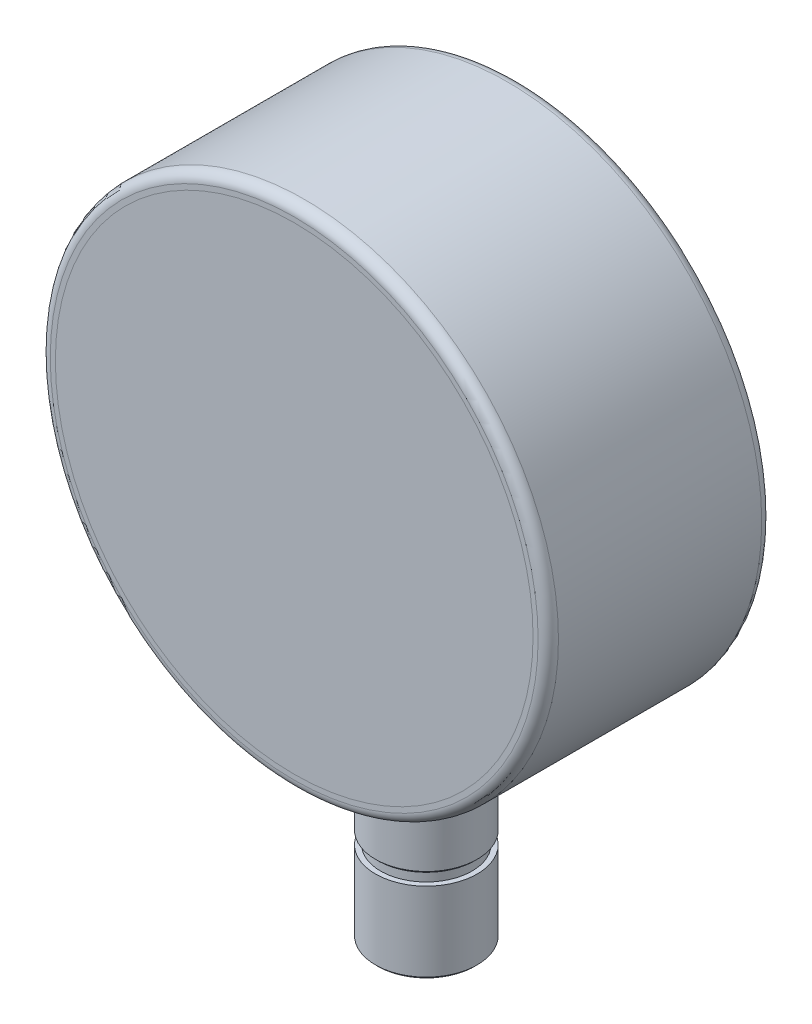
SolidWorks part; units mm, degrees
material "黄铜"
ref_plane "前视基准面" through (0, 0, 0) normal (0, 0, 1) x (1, 0, 0)
ref_plane "上视基准面" through (0, 0, 0) normal (0, 1, 0) x (1, 0, 0)
ref_plane "右视基准面" through (0, 0, 0) normal (1, 0, 0) x (0, 0, -1)
sketch "草图1" plane through (0, 0, 0) normal (0, 0, 1) x (1, 0, 0)
  circle A0 centre (0, 0) radius 50
  dimension "D" = 100
extrude "凸台-拉伸1" add sketch "草图1" along normal blind 44
fillet "圆角1" radius 2 2 edges at (50, 0, 44) (50, 0, 0)
ref_plane "基准面1" through (0, 0, 18) normal (0, 0, -1) x (-1, 0, 0)
sketch "草图2" plane through (0, 0, 18) normal (0, 0, -1) x (-1, 0, 0)
  line L0 (0, 0) -> (0, -90) construction
  line L1 (0, 0) -> (10, 0)
  line L2 (10, 0) -> (10, -70)
  line L3 (10, -70) -> (9, -70)
  line L4 (9, -70) -> (9, -72)
  line L5 (9, -72) -> (10, -72)
  line L6 (10, -72) -> (10, -88)
  line L7 (10, -88) -> (3, -88)
  line L8 (3, -88) -> (3, -90)
  line L9 (3, -90) -> (0, -90)
  line L10 (0, 0) -> (0, -90)
  dimension "B" = 90
  dimension "L" = 20
  dimension "L1" = 2
  dimension "d1" = 6
  dimension "D2" = 1
  dimension "(d)" = 20
  dimension "D3" = 2
revolve "旋转1" add sketch "草图2" angle 360 about L0
cosmetic thread "装饰螺纹线1" parameters "D2"=1
chamfer "倒角1" distance 0.5 angle 45 2 edges at (-10, -88, 18) (-10, -70, 18)
sketch "草图3" plane through (0, 0, 44) normal (0, 0, 1) x (1, 0, 0)
  circle A0 centre (0, 0) radius 47
  dimension "D1" = 94
extrude "切除-拉伸1" cut sketch "草图3" against normal blind 41
sketch "草图4" plane through (0, 0, 3) normal (0, 0, 1) x (1, 0, 0)
  line L0 (0, 0) -> (0, 45) construction
  line L1 (0, 0) -> (0, -45) construction
  line L2 (0, 0) -> (31.8198, -31.8198) construction
  line L3 (0, 0) -> (41.5746, 17.2208) construction
  line L4 (25.1456, -25.782) -> (31.5, -32.1364)
  line L5 (25.1456, -25.782) -> (25.782, -25.1456)
  line L6 (25.782, -25.1456) -> (32.1364, -31.5)
  line L7 (0, 0) -> (39.6865, -21.2129) construction
  line L8 (31.5, -32.1364) -> (31.8182, -31.8182)
  line L9 (39.6865, -21.2129) -> (39.7987, -21.0015)
  line L10 (39.7987, -21.0015) -> (35.0296, -18.4686)
  line L11 (35.0296, -18.4686) -> (34.8175, -18.8655)
  line L12 (39.6865, -21.2129) -> (39.5731, -21.4237)
  line L13 (39.5731, -21.4237) -> (34.8175, -18.8655)
  line L14 (0, 0) -> (36.1443, -26.8065) construction
  line L15 (33.1183, -24.8423) -> (33.3864, -24.4809)
  line L16 (33.3864, -24.4809) -> (36.2779, -26.6254)
  line L17 (36.2779, -26.6254) -> (36.1443, -26.8065)
  line L18 (36.0099, -26.9869) -> (36.1443, -26.8065)
  line L19 (33.1183, -24.8423) -> (36.0099, -26.9869)
  line L20 (39.0552, -13.7352) -> (42.4448, -14.948)
  line L21 (42.4448, -14.948) -> (42.3695, -15.16)
  line L22 (42.2932, -15.3717) -> (42.3695, -15.16)
  line L23 (38.9036, -14.1589) -> (42.2932, -15.3717)
  line L24 (39.0552, -13.7352) -> (38.9036, -14.1589)
  line L25 (0, 0) -> (38.9794, -13.9471) construction
  line L26 (41.3606, -1.8066) -> (44.9563, -1.9833)
  line L27 (44.9563, -1.9833) -> (44.9458, -2.208)
  line L28 (44.9342, -2.4327) -> (44.9458, -2.208)
  line L29 (41.3385, -2.2561) -> (44.9342, -2.4327)
  line L30 (41.3606, -1.8066) -> (41.3385, -2.2561)
  line L31 (44.1814, -8.5442) -> (38.8824, -7.5048)
  line L32 (44.1353, -8.7791) -> (44.1814, -8.5442)
  line L33 (38.7946, -7.9461) -> (38.8824, -7.5048)
  line L34 (44.088, -9.0137) -> (38.7946, -7.9461)
  line L35 (44.1353, -8.7791) -> (44.088, -9.0137)
  line L36 (0, 0) -> (41.3496, -2.0314) construction
  line L37 (40.2134, 9.841) -> (40.1041, 10.2775)
  line L38 (40.1041, 10.2775) -> (43.5962, 11.1522)
  line L39 (43.5962, 11.1522) -> (43.6514, 10.9341)
  line L40 (43.7055, 10.7157) -> (43.6514, 10.9341)
  line L41 (40.2134, 9.841) -> (43.7055, 10.7157)
  line L42 (44.7833, 4.4108) -> (44.7592, 4.6489)
  line L43 (44.7592, 4.6489) -> (39.3866, 4.1053)
  line L44 (39.3866, 4.1053) -> (39.4308, 3.6575)
  line L45 (44.7833, 4.4108) -> (44.8061, 4.1725)
  line L46 (44.8061, 4.1725) -> (39.4308, 3.6575)
  line L47 (0, 0) -> (38.8385, -7.7255) construction
  line L48 (41.4003, 17.6356) -> (41.7447, 16.8041)
  line L49 (33.4423, 13.3652) -> (41.7447, 16.8041)
  line L50 (33.0979, 14.1967) -> (33.4423, 13.3652)
  line L51 (33.0979, 14.1967) -> (41.4003, 17.6356)
  line L52 (33.4423, 13.3652) -> (41.7447, 16.8041)
  line L53 (33.0979, 14.1967) -> (41.4003, 17.6356)
  line L54 (34.6331, 28.7323) -> (30.468, 25.2955)
  line L55 (34.7855, 28.5477) -> (34.6331, 28.7323)
  line L56 (30.7535, 24.9477) -> (30.468, 25.2955)
  line L57 (34.9368, 28.3623) -> (30.7535, 24.9477)
  line L58 (34.7855, 28.5477) -> (34.9368, 28.3623)
  line L59 (35.3938, 21.4766) -> (38.4816, 23.3273)
  line L60 (38.4816, 23.3273) -> (38.5978, 23.1346)
  line L61 (38.713, 22.9413) -> (38.5978, 23.1346)
  line L62 (35.6252, 21.0906) -> (38.713, 22.9413)
  line L63 (35.3938, 21.4766) -> (35.6252, 21.0906)
  line L64 (25.0007, 37.4161) -> (24.8013, 37.5486)
  line L65 (24.8013, 37.5486) -> (21.8132, 33.0507)
  line L66 (21.8132, 33.0507) -> (22.1873, 32.8007)
  line L67 (25.0007, 37.4161) -> (25.1993, 37.2826)
  line L68 (25.1993, 37.2826) -> (22.1873, 32.8007)
  line L69 (27.9689, 30.5239) -> (27.6354, 30.8261)
  line L70 (27.6354, 30.8261) -> (30.0531, 33.4935)
  line L71 (30.0531, 33.4935) -> (30.2202, 33.3428)
  line L72 (30.3865, 33.1913) -> (30.2202, 33.3428)
  line L73 (27.9689, 30.5239) -> (30.3865, 33.1913)
  line L74 (17.9039, 37.3284) -> (17.4971, 37.5208)
  line L75 (17.4971, 37.5208) -> (19.0363, 40.7752)
  line L76 (19.0363, 40.7752) -> (19.24, 40.6795)
  line L77 (19.4431, 40.5828) -> (19.24, 40.6795)
  line L78 (17.9039, 37.3284) -> (19.4431, 40.5828)
  line L79 (5.852, 40.9844) -> (6.3802, 44.5454)
  line L80 (6.3802, 44.5454) -> (6.6029, 44.5129)
  line L81 (6.8254, 44.4794) -> (6.6029, 44.5129)
  line L82 (6.2971, 40.9183) -> (6.8254, 44.4794)
  line L83 (5.852, 40.9844) -> (6.2971, 40.9183)
  line L84 (12.8336, 43.1312) -> (11.2798, 37.9596)
  line L85 (13.0628, 43.0623) -> (12.8336, 43.1312)
  line L86 (11.7104, 37.8289) -> (11.2798, 37.9596)
  line L87 (13.2917, 42.9922) -> (11.7104, 37.8289)
  line L88 (13.0628, 43.0623) -> (13.2917, 42.9922)
  line L89 (-0.45, 44.9977) -> (0.45, 44.9977)
  line L90 (0.45, 36.0113) -> (0.45, 44.9977)
  line L91 (-0.45, 36.0113) -> (0.45, 36.0113)
  line L92 (-0.45, 36.0113) -> (-0.45, 44.9977)
  line L93 (-44.1353, -8.7791) -> (-44.088, -9.0137)
  line L94 (-44.088, -9.0137) -> (-38.7946, -7.9461)
  line L95 (-38.7946, -7.9461) -> (-38.8824, -7.5048)
  line L96 (-44.1353, -8.7791) -> (-44.1814, -8.5442)
  line L97 (-44.1814, -8.5442) -> (-38.8824, -7.5048)
  line L98 (-41.3606, -1.8066) -> (-41.3385, -2.2561)
  line L99 (-41.3385, -2.2561) -> (-44.9342, -2.4327)
  line L100 (-44.9342, -2.4327) -> (-44.9458, -2.208)
  line L101 (-44.9563, -1.9833) -> (-44.9458, -2.208)
  line L102 (-41.3606, -1.8066) -> (-44.9563, -1.9833)
  line L103 (-39.0552, -13.7352) -> (-38.9036, -14.1589)
  line L104 (-38.9036, -14.1589) -> (-42.2932, -15.3717)
  line L105 (-42.2932, -15.3717) -> (-42.3695, -15.16)
  line L106 (-42.4448, -14.948) -> (-42.3695, -15.16)
  line L107 (-39.0552, -13.7352) -> (-42.4448, -14.948)
  line L108 (-33.1183, -24.8423) -> (-36.0099, -26.9869)
  line L109 (-36.0099, -26.9869) -> (-36.1443, -26.8065)
  line L110 (-36.2779, -26.6254) -> (-36.1443, -26.8065)
  line L111 (-33.3864, -24.4809) -> (-36.2779, -26.6254)
  line L112 (-33.1183, -24.8423) -> (-33.3864, -24.4809)
  line L113 (-39.5731, -21.4237) -> (-34.8175, -18.8655)
  line L114 (-39.6865, -21.2129) -> (-39.5731, -21.4237)
  line L115 (-35.0296, -18.4686) -> (-34.8175, -18.8655)
  line L116 (-39.7987, -21.0015) -> (-35.0296, -18.4686)
  line L117 (-39.6865, -21.2129) -> (-39.7987, -21.0015)
  line L118 (-31.5, -32.1364) -> (-32.1364, -31.5)
  line L119 (-25.782, -25.1456) -> (-32.1364, -31.5)
  line L120 (-25.1456, -25.782) -> (-25.782, -25.1456)
  line L121 (-25.1456, -25.782) -> (-31.5, -32.1364)
  line L122 (-27.9689, 30.5239) -> (-30.3865, 33.1913)
  line L123 (-30.3865, 33.1913) -> (-30.2202, 33.3428)
  line L124 (-30.0531, 33.4935) -> (-30.2202, 33.3428)
  line L125 (-27.6354, 30.8261) -> (-30.0531, 33.4935)
  line L126 (-27.9689, 30.5239) -> (-27.6354, 30.8261)
  line L127 (-35.3938, 21.4766) -> (-35.6252, 21.0906)
  line L128 (-35.6252, 21.0906) -> (-38.713, 22.9413)
  line L129 (-38.713, 22.9413) -> (-38.5978, 23.1346)
  line L130 (-38.4816, 23.3273) -> (-38.5978, 23.1346)
  line L131 (-35.3938, 21.4766) -> (-38.4816, 23.3273)
  line L132 (-34.7855, 28.5477) -> (-34.9368, 28.3623)
  line L133 (-34.9368, 28.3623) -> (-30.7535, 24.9477)
  line L134 (-30.7535, 24.9477) -> (-30.468, 25.2955)
  line L135 (-34.7855, 28.5477) -> (-34.6331, 28.7323)
  line L136 (-34.6331, 28.7323) -> (-30.468, 25.2955)
  line L137 (-33.0979, 14.1967) -> (-41.4003, 17.6356)
  line L138 (-33.4423, 13.3652) -> (-41.7447, 16.8041)
  line L139 (-33.0979, 14.1967) -> (-41.4003, 17.6356)
  line L140 (-33.0979, 14.1967) -> (-33.4423, 13.3652)
  line L141 (-33.4423, 13.3652) -> (-41.7447, 16.8041)
  line L142 (-41.4003, 17.6356) -> (-41.7447, 16.8041)
  line L143 (-44.8061, 4.1725) -> (-39.4308, 3.6575)
  line L144 (-44.7833, 4.4108) -> (-44.8061, 4.1725)
  line L145 (-39.3866, 4.1053) -> (-39.4308, 3.6575)
  line L146 (-44.7592, 4.6489) -> (-39.3866, 4.1053)
  line L147 (-44.7833, 4.4108) -> (-44.7592, 4.6489)
  line L148 (-40.2134, 9.841) -> (-43.7055, 10.7157)
  line L149 (-43.7055, 10.7157) -> (-43.6514, 10.9341)
  line L150 (-43.5962, 11.1522) -> (-43.6514, 10.9341)
  line L151 (-40.1041, 10.2775) -> (-43.5962, 11.1522)
  line L152 (-40.2134, 9.841) -> (-40.1041, 10.2775)
  line L153 (-17.9039, 37.3284) -> (-19.4431, 40.5828)
  line L154 (-19.4431, 40.5828) -> (-19.24, 40.6795)
  line L155 (-19.0363, 40.7752) -> (-19.24, 40.6795)
  line L156 (-17.4971, 37.5208) -> (-19.0363, 40.7752)
  line L157 (-17.9039, 37.3284) -> (-17.4971, 37.5208)
  line L158 (-25.1993, 37.2826) -> (-22.1873, 32.8007)
  line L159 (-25.0007, 37.4161) -> (-25.1993, 37.2826)
  line L160 (-21.8132, 33.0507) -> (-22.1873, 32.8007)
  line L161 (-24.8013, 37.5486) -> (-21.8132, 33.0507)
  line L162 (-25.0007, 37.4161) -> (-24.8013, 37.5486)
  line L163 (-13.0628, 43.0623) -> (-13.2917, 42.9922)
  line L164 (-13.2917, 42.9922) -> (-11.7104, 37.8289)
  line L165 (-11.7104, 37.8289) -> (-11.2798, 37.9596)
  line L166 (-13.0628, 43.0623) -> (-12.8336, 43.1312)
  line L167 (-12.8336, 43.1312) -> (-11.2798, 37.9596)
  line L168 (-5.852, 40.9844) -> (-6.2971, 40.9183)
  line L169 (-6.2971, 40.9183) -> (-6.8254, 44.4794)
  line L170 (-6.8254, 44.4794) -> (-6.6029, 44.5129)
  line L171 (-6.3802, 44.5454) -> (-6.6029, 44.5129)
  line L172 (-5.852, 40.9844) -> (-6.3802, 44.5454)
  circle A0 centre (0, 0) radius 45 construction
  point P18 (34.9235, -18.667)
  point P23 (33.2523, -24.6616)
  point P28 (38.9794, -13.9471)
  point P35 (41.3496, -2.0314)
  point P41 (38.8385, -7.7255)
  point P48 (40.1587, 10.0592)
  point P54 (39.4087, 3.8814)
  point P99 (30.6107, 25.1216)
  point P100 (35.5095, 21.2836)
  point P101 (22.0002, 32.9257)
  point P102 (27.8022, 30.675)
  point P103 (17.7005, 37.4246)
  point P104 (6.0746, 40.9514)
  point P105 (11.4951, 37.8942)
  point P137 (-38.8385, -7.7255)
  point P138 (-41.3496, -2.0314)
  point P139 (-38.9794, -13.9471)
  point P140 (-33.2523, -24.6616)
  point P141 (-34.9235, -18.667)
  point P171 (-27.8022, 30.675)
  point P172 (-35.5095, 21.2836)
  point P173 (-30.6107, 25.1216)
  point P174 (-39.4087, 3.8814)
  point P175 (-40.1587, 10.0592)
  point P186 (-17.7005, 37.4246)
  point P187 (-22.0002, 32.9257)
  point P198 (-11.4951, 37.8942)
  point P199 (-6.0746, 40.9514)
  dimension "D1" = 90
  dimension "D2" = 45
  dimension "D4" = 0.9
  dimension "D5" = 9
  dimension "D6" = 16.875
  dimension "D7" = 0.45
  dimension "D8" = 5.4
  dimension "D9" = 8.438
  dimension "D10" = 0.45
  dimension "D11" = 3.6
extrude "凸台-拉伸2" add sketch "草图4" along normal blind 1 contours L15 L19 L18 L17 L16 | L13 L12 L9 L10 L11 | L20 L24 L23 L22 L21 | L35 L32 L31 L33 L34 | L26 L30 L29 L28 L27 | L46 L45 L42 L43 L44 | L37 L41 L40 L39 L38 | L51 L50 L49 L48 | L59 L63 L62 L61 L60 | L58 L55 L54 L56 L57 | L69 L73 L72 L71 L70 | L68 L67 L64 L65 L66 | L74 L78 L77 L76 L75 | L88 L85 L84 L86 L87 | L79 L83 L82 L81 L80 | L92 L91 L90 L89 | L168 L172 L171 L170 L169 | L167 L166 L163 L164 L165 | L153 L157 L156 L155 L154 | L162 L159 L158 L160 L161 | L122 L126 L125 L124 L123 | L136 L135 L132 L133 L134 | L127 L131 L130 L129 L128 | L137 L142 L138 L140 | L148 L152 L151 L150 L149 | L147 L144 L143 L145 L146 | L98 L102 L101 L100 L99 | L97 L96 L93 L94 L95 | L103 L107 L106 L105 L104 | L117 L114 L113 L115 L116 | L108 L112 L111 L110 L109 | L121 L120 L119 L118
mirror "镜向1" about plane through (0, 0, 0) normal (1, 0, 0) of "凸台-拉伸2"
sketch "草图5" plane through (0, 0, 3) normal (0, 0, 1) x (1, 0, 0)
  circle A0 centre (0, 0) radius 2
  dimension "D1" = 4
extrude "凸台-拉伸3" add sketch "草图5" along normal blind 3
fillet "圆角2" radius 1 1 edges at (2, 0, 6)
sketch "草图6" plane through (0, 0, 3) normal (0, 0, 1) x (1, 0, 0)
  line L0 (0, 0) -> (-23, -39.8372) construction
  line L1 (0, 0) -> (0, -46) construction
  line L2 (2.6545, 1.3977) -> (6.7583, 5.7748)
  line L3 (-23, -39.8372) -> (-2.6785, -1.3512)
  line L4 (-23, -39.8372) -> (0.169, -2.9952)
  line L5 (-0.1168, 2.9977) -> (1.6219, 8.7403)
  line L6 (0, 0) -> (6, 10.3923) construction
  line L7 (7.1225, 9.7442) -> (4.8775, 11.0404)
  arc A0 (0.169, -2.9952) -> (2.6545, 1.3977) centre (0, 0) ccw
  circle A1 centre (0, 0) radius 2
  circle A2 centre (0, 0) radius 2 construction
  arc A3 (7.1108, 6.0526) -> (6.7583, 5.7748) centre (7.8526, 4.7488) ccw
  arc A4 (7.1108, 6.0526) -> (7.1225, 9.7442) centre (6.0588, 7.9017) ccw
  circle A5 centre (0, 0) radius 2
  arc A6 (1.6863, 9.1844) -> (1.6219, 8.7403) centre (0.1863, 9.175) cw
  arc A7 (1.6863, 9.1844) -> (4.8775, 11.0404) centre (3.8137, 9.1979) cw
  circle A8 centre (0, 0) radius 46 construction
  arc A9 (-0.1168, 2.9977) -> (-2.6785, -1.3512) centre (0, 0) ccw
  dimension "D2" = 92
  dimension "D6" = 3
  dimension "D7" = 12
  dimension "D10" = 2.1275
  dimension "D4" = 3.2
  dimension "D1" = 6
  dimension "D3" = 30
  dimension "D5" = 3.288
  dimension "D8" = 6
  dimension "D9" = 5.931
extrude "凸台-拉伸4" add sketch "草图6" along normal blind 2 contours L5 A9 L3 L4 A0 L2 A3 A4 L7 A7 A6 A1
sketch "草图7" plane through (0, 0, 3) normal (0, 0, 1) x (1, 0, 0)
  line L0 (0, 0) -> (22.8012, 24.8831) construction
  line L1 (0, 0) -> (32.1879, 10.1488) construction
  line L2 (0, 0) -> (31.7146, -11.5432) construction
  line L3 (0, 0) -> (-11.5432, 31.7146) construction
  line L4 (0, 0) -> (5.8606, 33.2373) construction
  line L5 (0, 0) -> (-29.9366, 15.584) construction
  line L6 (0, 0) -> (-33.7179, -1.4722) construction
  line L7 (0, 0) -> (-25.854, -21.6941) construction
  line L8 (0, 0) -> (-21.6941, -25.854) construction
  line L9 (0, 0) -> (25.4638, -25.4638) construction
  line L10 (25.1456, -25.782) -> (25.782, -25.1456) construction
  line L11 (0, 0) -> (33.2701, 13.7809) construction
  line L12 (0, 0) -> (-33.2701, 13.7809) construction
  line L13 (-33.2701, 13.7809) -> (-31.1875, 12.9183) construction
  line L14 (0, 0) -> (21.6941, -25.854) construction
  line L15 (23.8649, -23.8649) -> (17.8649, -23.8649) construction
  line L16 (33.0979, 14.1967) -> (33.4423, 13.3652) construction
  line L17 (0, 0) -> (0, 36.0113) construction
  line L18 (-0.45, 36.0113) -> (0.45, 36.0113) construction
  line L19 (-33.0979, 14.1967) -> (-33.4423, 13.3652) construction
  line L20 (27.4423, 10.3652) -> (33.4423, 10.3652) construction
  line L21 (3, 32.0113) -> (-3, 32.0113) construction
  line L22 (-29.389, 10.3652) -> (-33.389, 10.3652) construction
  line L23 (0, 0) -> (-23.8649, -23.8649) construction
  line L24 (0, 0) -> (0, -47) construction
  line L25 (-23.8649, -23.8649) -> (-17.8649, -23.8649) construction
  line L26 (-0.45, 36.0113) -> (0.45, 36.0113) construction
  line L27 (-33.2701, 13.7809) -> (-33.75, 0) construction
  line L28 (33.4423, 13.3652) -> (33.4423, 1.0755) construction
  arc A0 (32.1879, 10.1488) -> (22.8012, 24.8831) centre (0, 0) ccw construction
  arc A1 (5.8606, 33.2373) -> (-11.5432, 31.7146) centre (0, 0) ccw construction
  arc A2 (-29.9366, 15.584) -> (-33.7179, -1.4722) centre (0, 0) ccw construction
  arc A3 (-25.854, -21.6941) -> (-21.6941, -25.854) centre (0, 0) ccw construction
  arc A4 (21.6941, -25.854) -> (31.7146, -11.5432) centre (0, 0) ccw construction
  circle A5 centre (0, 0) radius 47 construction
  text T0 "0" font "Century Gothic" height in points 8
  text T1 "1.6" font "Century Gothic" height in points 8
  text T2 "1.2" font "Century Gothic" height in points 8
  text T3 "0.8" font "Century Gothic" height in points 8
  text T4 "0.4" font "Century Gothic" height in points 8
  dimension "D1" = 67.5
  dimension "D2" = 30
  dimension "D3" = 25
  dimension "D4" = 5
  dimension "D5" = 30
  dimension "D6" = 20
  dimension "D7" = 30
  dimension "D8" = 30
  dimension "D9" = 5
  dimension "D10" = 45
  dimension "D11" = 5
  dimension "D12" = 6
  dimension "D13" = 6
  dimension "D14" = 3
  dimension "D15" = 3
  dimension "D16" = 6
  dimension "D17" = 4
  dimension "D18" = 4
  dimension "D19" = 6
extrude "凸台-拉伸8" add sketch "草图7" along normal blind 2
ref_plane "基准面2" through (0, 0, 44) normal (0, 0, 1) x (1, 0, 0)
sketch "草图8" plane through (0, 0, 44) normal (0, 0, 1) x (1, 0, 0)
  circle A0 centre (0, 0) radius 47
  circle A1 centre (0, 0) radius 47 construction
extrude "凸台-拉伸7" add sketch "草图8" against normal blind 2 separate body
